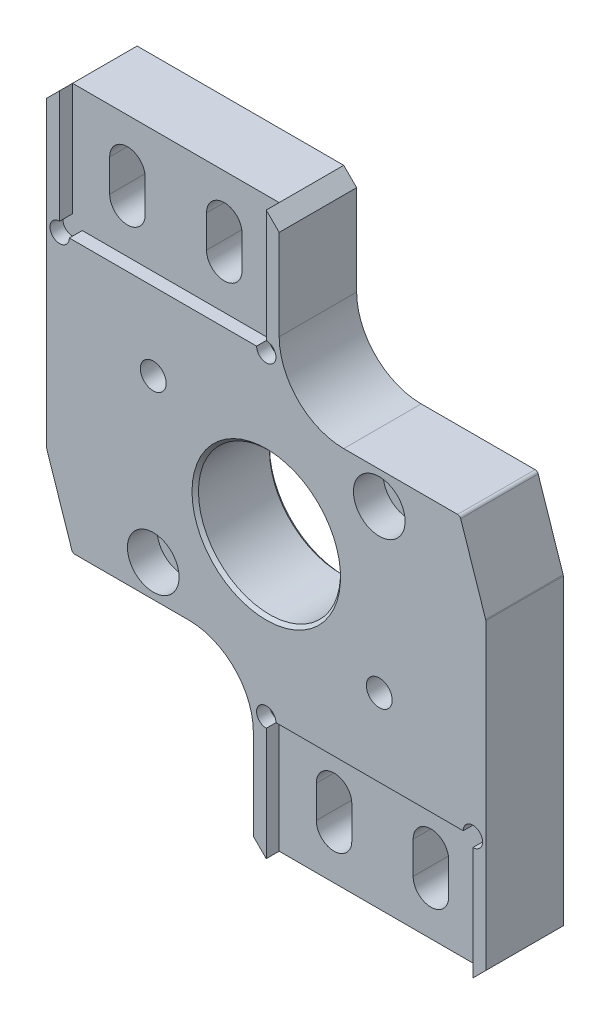
from build123d import *
from OCP.BRepFilletAPI import BRepFilletAPI_MakeChamfer

# Parameters (mm, degrees)
SKETCH1_W                                            = 68
SKETCH1_H                                            = 87
BOSS_EXTRUDE1_DEPTH                                  = 12
SKETCH3_R                                            = 11
SKETCH3_R_2                                          = 2
SKETCH3_W                                            = 32
SKETCH3_H                                            = 26
CUT_EXTRUDE2_DEPTH                                   = 57.5
FILLET1_R                                            = 10
CHAMFER1_SIZE                                        = 2
CHAMFER2_SIZE                                        = 4
CHAMFER2_SIZE2                                       = 12
FILLET3_R                                            = 0.5
CUT_EXTRUDE4_DEPTH                                   = 57.5
HOLE_SIZE_BY_SOCKET_HEAD_CAP_SCREW_TYPE0_D           = 4.5
HOLE_SIZE_BY_SOCKET_HEAD_CAP_SCREW_TYPE0_CBORE_D     = 8
HOLE_SIZE_BY_SOCKET_HEAD_CAP_SCREW_TYPE0_CBORE_DEPTH = 4.6
CHAMFER3_SIZE                                        = 0.5
CUT_EXTRUDE3_DEPTH                                   = 2


with BuildPart() as part:
    # Sketch1 → Boss-Extrude1 (new body)
    with BuildSketch(Plane.XY):
        Rectangle(SKETCH1_W, SKETCH1_H)
    extrude(amount=BOSS_EXTRUDE1_DEPTH)

    # Sketch3 → Cut-Extrude2 (cut, through all)
    with BuildSketch(Plane.XY.offset(12)):
        Circle(SKETCH3_R)
        with Locations((17.5, -12.5)):
            Circle(SKETCH3_R_2)
        with Locations((-17.5, 12.5)):
            Circle(SKETCH3_R_2)
        with Locations((18, 30.5)):
            Rectangle(SKETCH3_W, SKETCH3_H)
        with Locations((-18, -30.5)):
            Rectangle(SKETCH3_W, SKETCH3_H)
    extrude(amount=-CUT_EXTRUDE2_DEPTH, mode=Mode.SUBTRACT)

    # Fillet1
    fillet1_edges = [part.edges().sort_by_distance(p)[0] for p in [
        (2, 17.5, 6),
        (-2, -17.5, 6),
    ]]
    fillet(fillet1_edges, radius=FILLET1_R)

    # Chamfer1
    chamfer1_edges = [part.edges().sort_by_distance(p)[0] for p in [
        (2, 43.5, 6),
        (-2, -43.5, 6),
        (34, -43.5, 6),
        (-34, 43.5, 6),
    ]]
    chamfer(chamfer1_edges, length=CHAMFER1_SIZE)

    # Chamfer2: one chamfer whose edges measure the first distance from different faces: ONE call of the kernel's chamfer builder (chamfer() names one face for all edges)
    chamfer2_edges_1 = [part.edges().sort_by_distance(p)[0] for p in [
        (34, 17.5, 6),
    ]]
    chamfer2_side_1 = [part.faces().sort_by_distance(p)[0] for p in [
        (23, 17.5, 6),
    ]]
    chamfer2_edges_2 = [part.edges().sort_by_distance(p)[0] for p in [
        (-34, -17.5, 6),
    ]]
    chamfer2_side_2 = [part.faces().sort_by_distance(p)[0] for p in [
        (-23, -17.5, 6),
    ]]
    chamfer2 = BRepFilletAPI_MakeChamfer(part.part.solid().wrapped)
    for e in chamfer2_edges_1:
        chamfer2.Add(CHAMFER2_SIZE, CHAMFER2_SIZE2, e.wrapped, chamfer2_side_1[0].wrapped)  # the first distance lies on this face
    for e in chamfer2_edges_2:
        chamfer2.Add(CHAMFER2_SIZE, CHAMFER2_SIZE2, e.wrapped, chamfer2_side_2[0].wrapped)  # the first distance lies on this face
    add(Compound.cast(chamfer2.Shape()), mode=Mode.REPLACE)

    # Fillet3
    fillet3_edges = [part.edges().sort_by_distance(p)[0] for p in [
        (-34, -5.5, 6),
        (-30, -17.5, 6),
        (34, 5.5, 6),
        (30, 17.5, 6),
    ]]
    fillet(fillet3_edges, radius=FILLET3_R)

    # Sketch21 → Cut-Extrude4 (cut, through all)
    with BuildSketch(Plane(origin=(0, 0, 0), x_dir=(-1, 0, 0), z_dir=(0, 0, -1))):
        with BuildLine():
            Line((11.25, 36.5), (11.25, 31.500000357))
            ThreePointArc((11.25, 31.500000357), (8.5, 28.750000357), (5.75, 31.500000357))
            Line((5.75, 31.500000357), (5.75, 36.5))
            ThreePointArc((5.75, 36.5), (8.5, 39.25), (11.25, 36.5))
        make_face()
        with BuildLine():
            Line((26.25, 36.500000178), (26.25, 31.500000178))
            ThreePointArc((26.25, 31.500000178), (23.5, 28.750000357), (20.75, 31.500000178))
            Line((20.75, 31.500000178), (20.75, 36.500000178))
            ThreePointArc((20.75, 36.500000178), (23.5, 39.25), (26.25, 36.500000178))
        make_face()
        with BuildLine():
            Line((-20.75, -31.500000357), (-20.75, -36.5))
            ThreePointArc((-20.75, -36.5), (-23.5, -39.25), (-26.25, -36.5))
            Line((-26.25, -36.5), (-26.25, -31.500000357))
            ThreePointArc((-26.25, -31.500000357), (-23.5, -28.750000357), (-20.75, -31.500000357))
        make_face()
        with BuildLine():
            Line((-5.75, -31.500000357), (-5.75, -36.5))
            ThreePointArc((-5.75, -36.5), (-8.5, -39.25), (-11.25, -36.5))
            Line((-11.25, -36.5), (-11.25, -31.500000357))
            ThreePointArc((-11.25, -31.500000357), (-8.5, -28.750000357), (-5.75, -31.500000357))
        make_face()
    extrude(amount=-CUT_EXTRUDE4_DEPTH, mode=Mode.SUBTRACT)

    # Hole size by socket head cap screw type0 (through all)
    with Locations(Plane.XY.offset(12)):
        with Locations((17.5, 12.5), (-17.5, -12.5)):
            CounterBoreHole(HOLE_SIZE_BY_SOCKET_HEAD_CAP_SCREW_TYPE0_D / 2, HOLE_SIZE_BY_SOCKET_HEAD_CAP_SCREW_TYPE0_CBORE_D / 2, HOLE_SIZE_BY_SOCKET_HEAD_CAP_SCREW_TYPE0_CBORE_DEPTH)

    # Chamfer3
    chamfer3_edges = [part.edges().sort_by_distance(p)[0] for p in [
        (-11, 0, 0),
        (-11, 0, 12),
    ]]
    chamfer(chamfer3_edges, length=CHAMFER3_SIZE)

    # Sketch19 → Cut-Extrude3 (cut)
    with BuildSketch(Plane.XY.offset(12)):
        with BuildLine():
            Line((32, -43.5), (0, -43.5))
            Line((0, -43.5), (0, -26))
            ThreePointArc((0, -26), (-1.060660172, -23.439339828), (1.5, -24.5))
            Line((1.5, -24.5), (30.5, -24.5))
            ThreePointArc((30.5, -24.5), (33.060660172, -23.439339828), (32, -26))
            Line((32, -26), (32, -43.5))
        make_face()
        with BuildLine():
            Line((0, 43.5), (-32, 43.5))
            Line((-32, 43.5), (-32, 26))
            ThreePointArc((-32, 26), (-33.060660172, 23.439339828), (-30.5, 24.5))
            Line((-30.5, 24.5), (-1.5, 24.5))
            ThreePointArc((-1.5, 24.5), (1.060660172, 23.439339828), (0, 26))
            Line((0, 26), (0, 43.5))
        make_face()
    extrude(amount=-CUT_EXTRUDE3_DEPTH, mode=Mode.SUBTRACT)


solid = part.part
